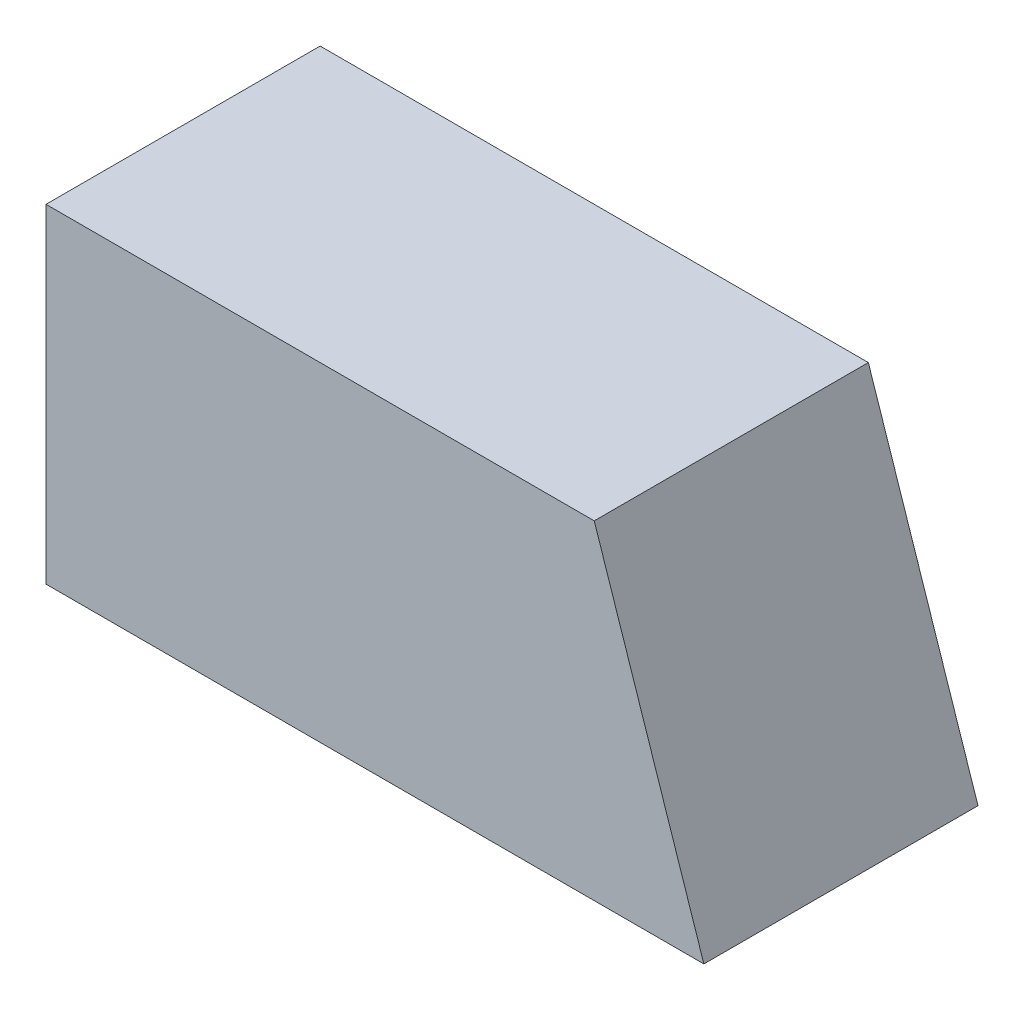
SolidWorks part; units mm, degrees
ref_plane "Front Plane" through (0, 0, 0) normal (0, 0, 1) x (1, 0, 0)
ref_plane "Top Plane" through (0, 0, 0) normal (0, 1, 0) x (1, 0, 0)
ref_plane "Right Plane" through (0, 0, 0) normal (1, 0, 0) x (0, 0, -1)
sketch "Sketch1" plane through (0, 0, 0) normal (0, 0, 1) x (1, 0, 0)
  line L0 (0, 0) -> (0, 600)
  line L1 (0, 600) -> (1000, 600)
  line L2 (1000, 600) -> (1200, 0)
  line L3 (1200, 0) -> (0, 0)
  dimension "D1" = 1000
  dimension "D2" = 1200
  dimension "D3" = 600
extrude "Boss-Extrude1" add sketch "Sketch1" along normal blind 500
